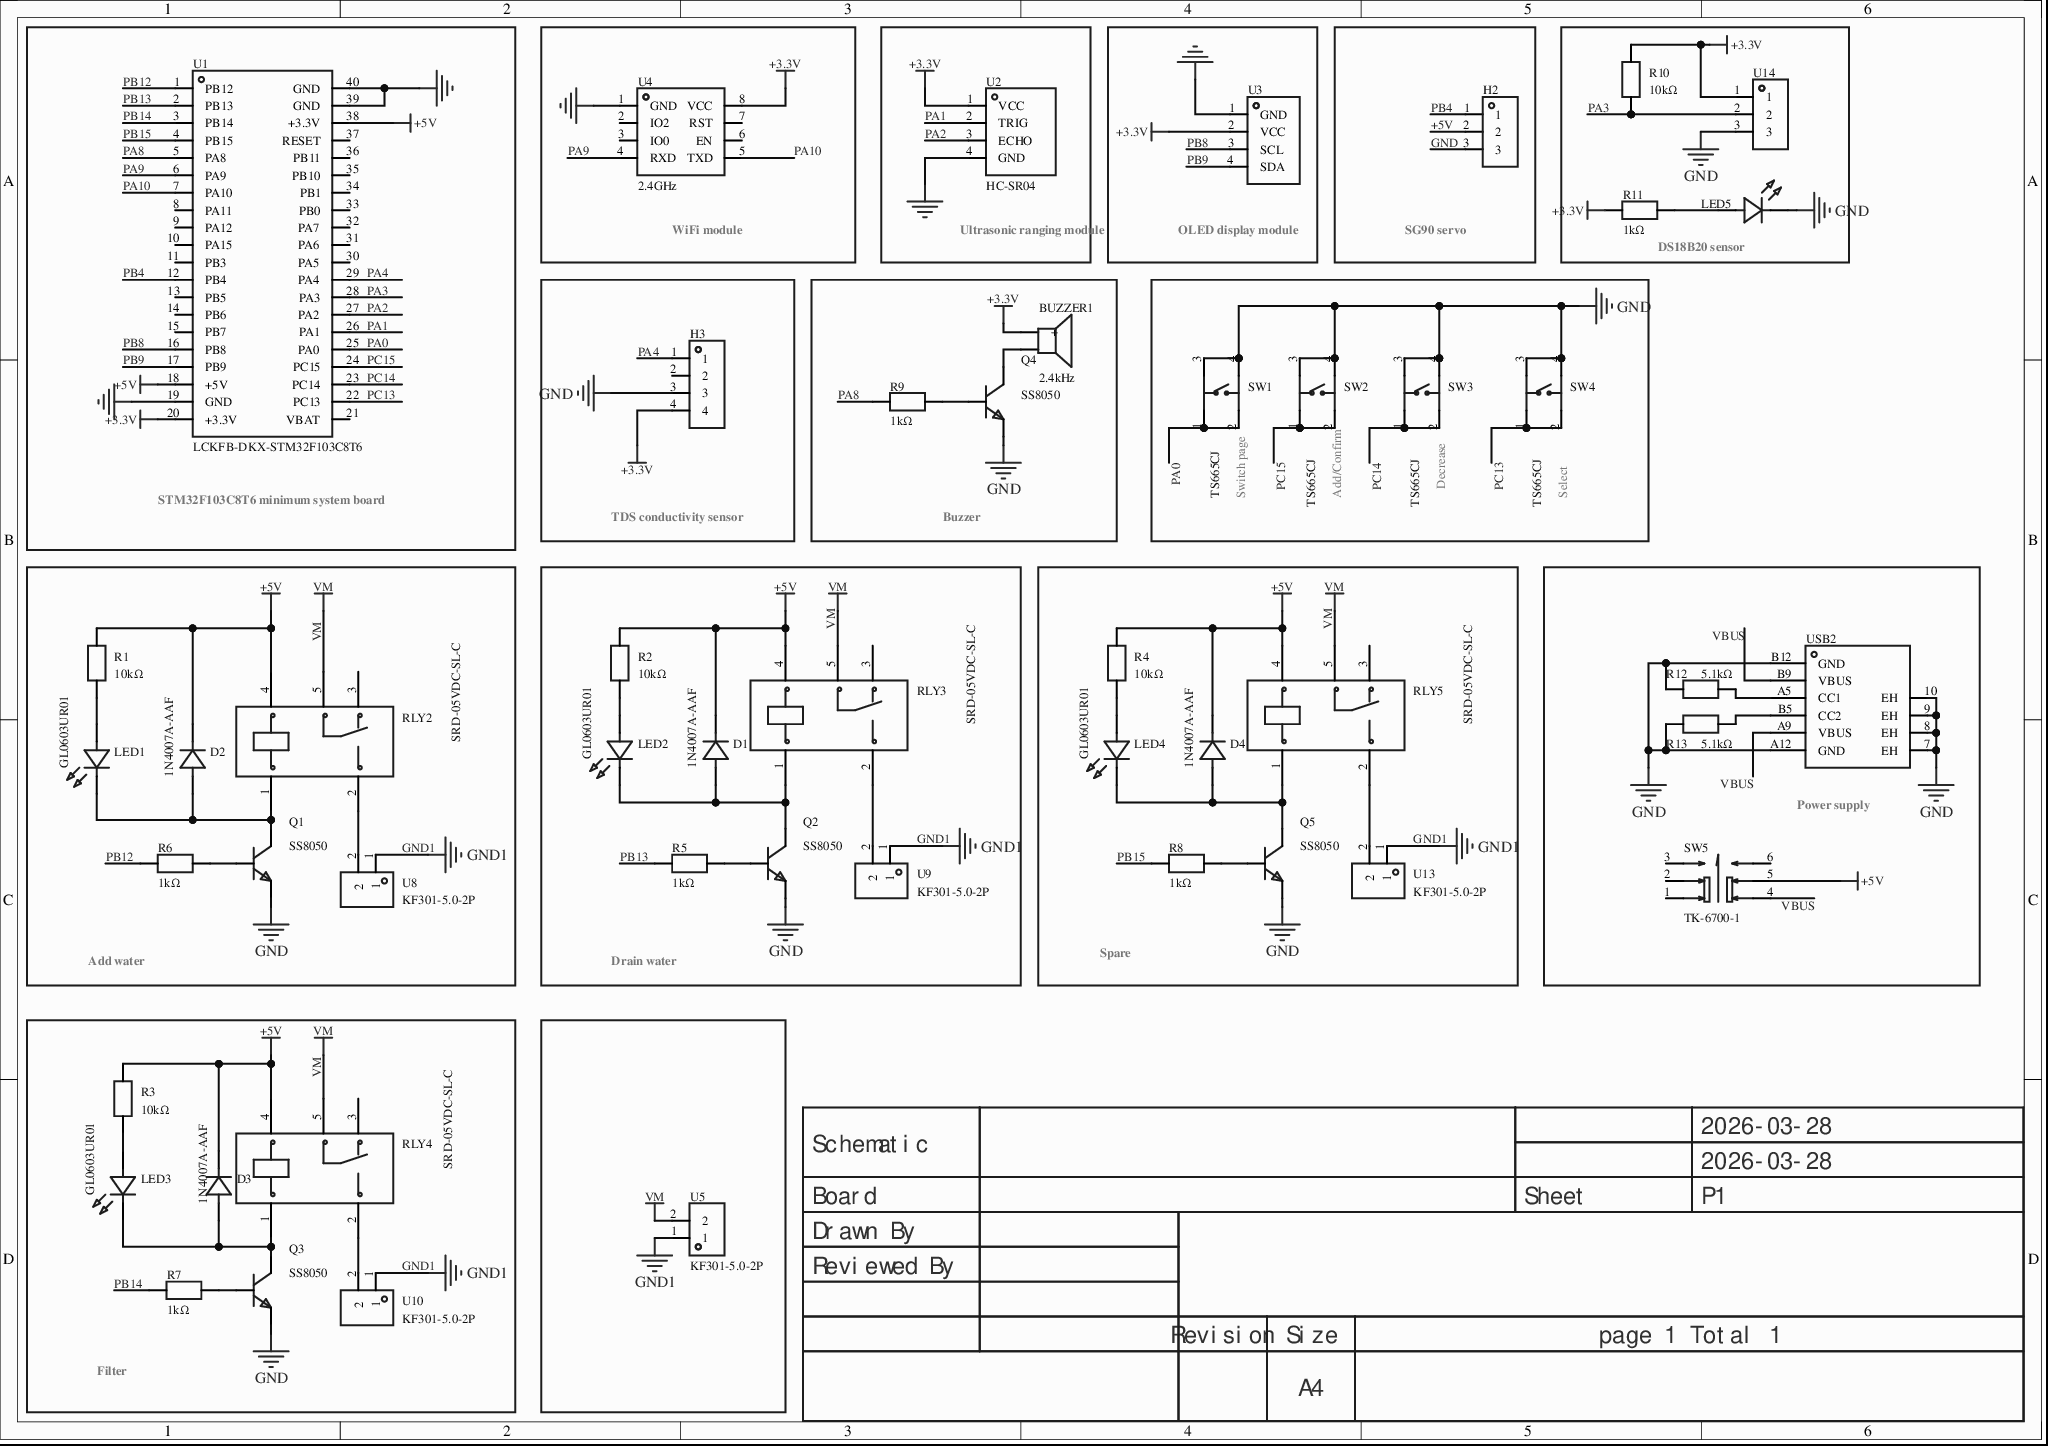
[diagram p0: MISC62342-3.schdoc]
# Altium project MISC62342-2.PrjPcb
1 sheet, 50 parts. Net scope: global (net labels, ports and power ports of the same name join across sheets).
Board file: MISC62342.pcbdoc

## Sheet MISC62342-3.schdoc
size 297 x 209 mm; Version: V1.0; @Project Name: MISC62342; @Page Count: 1; @Update Date: 2026-03-28; @Create Date: 2026-03-28; @Schematic Name: MISC62342; @Page No: 1; @Board Name: MISC62342; @Create Time: 18:09:04; @Update Time: 20:53:11; Size: A4

### Parts
BUZZER1  2.4kHz  [BUZ-TH_BD12.0-P7.60-D0.6-FD]
D1  1N4007A-AAF  [SMA_L4.3-W2.6-LS5.0-RD]
D2  1N4007A-AAF  [SMA_L4.3-W2.6-LS5.0-RD]
D3  1N4007A-AAF  [SMA_L4.3-W2.6-LS5.0-RD]
D4  1N4007A-AAF  [SMA_L4.3-W2.6-LS5.0-RD]
H2  PZ254V-11-03P  [HDR-TH_3P-P2.54-V-M_PZ254V-11-03P]  (value not drawn)
H3  PZ254V-11-04P  [HDR-TH_4P-P2.54-V-M]  (value not drawn)
LED1  GL0603UR01  [LED0603-FD]
LED2  GL0603UR01  [LED0603-FD]
LED3  GL0603UR01  [LED0603-FD]
LED4  GL0603UR01  [LED0603-FD]
LED5  GL0603UR01  [LED0603-FD]  (value not drawn)
Q1  SS8050  [SOT-23-3_L2.9-W1.3-P1.90-LS2.4-BR]
Q2  SS8050  [SOT-23-3_L2.9-W1.3-P1.90-LS2.4-BR]
Q3  SS8050  [SOT-23-3_L2.9-W1.3-P1.90-LS2.4-BR]
Q4  SS8050  [SOT-23-3_L2.9-W1.3-P1.90-LS2.4-BR]
Q5  SS8050  [SOT-23-3_L2.9-W1.3-P1.90-LS2.4-BR]
R1  10kΩ  [RES-TH_BD2.7-L6.2-P10.20-D0.4]
R2  10kΩ  [RES-TH_BD2.7-L6.2-P10.20-D0.4]
R3  10kΩ  [RES-TH_BD2.7-L6.2-P10.20-D0.4]
R4  10kΩ  [RES-TH_BD2.7-L6.2-P10.20-D0.4]
R5  1kΩ  [RES-TH_BD2.7-L6.2-P10.20-D0.4]
R6  1kΩ  [RES-TH_BD2.7-L6.2-P10.20-D0.4]
R7  1kΩ  [RES-TH_BD2.7-L6.2-P10.20-D0.4]
R8  1kΩ  [RES-TH_BD2.7-L6.2-P10.20-D0.4]
R9  1kΩ  [RES-TH_BD2.7-L6.2-P10.20-D0.4]
R10  10kΩ  [RES-TH_BD2.7-L6.2-P10.20-D0.4]
R11  1kΩ  [RES-TH_BD2.7-L6.2-P10.20-D0.4]
R12  5.1kΩ  [RES-TH_BD2.7-L6.2-P10.20-D0.4]
R13  5.1kΩ  [RES-TH_BD2.7-L6.2-P10.20-D0.4]
RLY2  SRD-05VDC-SL-C  [RELAY-TH_SRD-XXVDC-XL-C]
RLY3  SRD-05VDC-SL-C  [RELAY-TH_SRD-XXVDC-XL-C]
RLY4  SRD-05VDC-SL-C  [RELAY-TH_SRD-XXVDC-XL-C]
RLY5  SRD-05VDC-SL-C  [RELAY-TH_SRD-XXVDC-XL-C]
SW1  TS665CJ  [SW-TH_4P-L6.0-W6.0-P4.50-LS6.5]
SW2  TS665CJ  [SW-TH_4P-L6.0-W6.0-P4.50-LS6.5]
SW3  TS665CJ  [SW-TH_4P-L6.0-W6.0-P4.50-LS6.5]
SW4  TS665CJ  [SW-TH_4P-L6.0-W6.0-P4.50-LS6.5]
SW5  TK-6700-1  [SW-TH_TK-6700-1]
U1  LCKFB-DKX-STM32F103C8T6  [CONN-TH_L53.3-W22.9_STM32F103C8T6-CARD]
U2  HC-SR04  [TH_HC-SR04V]
U3  HS96L03W2C03  [OLED-TH_L27.8-W27.2-P2.54_C9900033791]  (value not drawn)
U4  2.4GHz  [WIFIM-TH_8P-L24.7-W14.4-P2.54]
U5  KF301-5.0-2P  [CONN-TH_P5.00_KF301-5.0-2P]
U8  KF301-5.0-2P  [CONN-TH_P5.00_KF301-5.0-2P]
U9  KF301-5.0-2P  [CONN-TH_P5.00_KF301-5.0-2P]
U10  KF301-5.0-2P  [CONN-TH_P5.00_KF301-5.0-2P]
U13  KF301-5.0-2P  [CONN-TH_P5.00_KF301-5.0-2P]
U14  WAFER-XH2.54-3PWZ  [CONN-TH_3P-P2.50_WAFER-XH2.54-3PWZ]  (value not drawn)
USB2  (no value)  [USB_ TYPE-C-6P]

### Blocks framed on the sheet
STM32F103C8T6 minimum system board: U1
WiFi module: U4
Ultrasonic ranging module: U2
OLED display module: U3
SG90 servo: H2
DS18B20 sensor: LED5 R10 R11 U14
TDS conductivity sensor: H3
Buzzer: BUZZER1 Q4 R9
Add water: D2 LED1 Q1 R1 R6 RLY2 U8
Drain water: D1 LED2 Q2 R2 R5 RLY3 U9
Spare: D4 LED4 Q5 R4 R8 RLY5 U13
Power supply: R12 R13 SW5 USB2
Filter: D3 LED3 Q3 R3 R7 RLY4 U10

### Nets
+3.3V: BUZZER1.1(+) H3.4 R10.2 R11.2 U1.20(+3.3V) U2.1(VCC) U3.2(VCC) U4.8(VCC) U14.1
+5V: D1.1(K) D2.1(K) D3.1(K) D4.1(K) H2.2 R1.2 R2.2 R3.2 R4.2 RLY2.4 RLY3.4 RLY4.4 RLY5.4 SW5.5 U1.18(+5V) U1.38(+3.3V)
GND: H2.3 H3.3 LED5.1(K) Q1.2(E) Q2.2(E) Q3.2(E) Q4.2(E) Q5.2(E) R12.1 R13.2 SW1.3(B) SW1.4(D) SW2.3(B) SW2.4(D) SW3.3(B) SW3.4(D) SW4.3(B) SW4.4(D) U1.19(GND) U1.39(GND) U1.40(GND) U2.4(GND) U3.1(GND) U4.1(GND) U14.3 USB2.7(EH) USB2.8(EH) USB2.9(EH) USB2.10(EH) USB2.A12(GND) USB2.B12(GND)
GND1: U5.1 U8.1 U9.1 U10.1 U13.1
VM: RLY2.5 RLY3.5 RLY4.5 RLY5.5 U5.2
PA0: SW1.1(A) SW1.2(C) U1.25(PA0)
PA1: U1.26(PA1) U2.2(TRIG)
PA2: U1.27(PA2) U2.3(ECHO)
PA3: R10.1 U1.28(PA3) U14.2
PA4: H3.1 U1.29(PA4)
PA8: R9.1 U1.5(PA8)
PA9: U1.6(PA9) U4.4(RXD)
PA10: U1.7(PA10) U4.5(TXD)
PB4: H2.1 U1.12(PB4)
PB8: U1.16(PB8) U3.3(SCL)
PB9: U1.17(PB9) U3.4(SDA)
PB12: R6.1 U1.1(PB12)
PB13: R5.1 U1.2(PB13)
PB14: R7.1 U1.3(PB14)
PB15: R8.1 U1.4(PB15)
PC13: SW4.1(A) SW4.2(C) U1.22(PC13)
PC14: SW3.1(A) SW3.2(C) U1.23(PC14)
PC15: SW2.1(A) SW2.2(C) U1.24(PC15)
VBUS: SW5.4 USB2.A9(VBUS) USB2.B9(VBUS)
NetBUZZER1_2: BUZZER1.2 Q4.3(C)
NetD1_2: D1.2(A) LED2.1(K) Q2.3(C) RLY3.1
NetD2_2: D2.2(A) LED1.1(K) Q1.3(C) RLY2.1
NetD3_2: D3.2(A) LED3.1(K) Q3.3(C) RLY4.1
NetD4_2: D4.2(A) LED4.1(K) Q5.3(C) RLY5.1
NetLED1_2: LED1.2(A) R1.1
NetLED2_2: LED2.2(A) R2.1
NetLED3_2: LED3.2(A) R3.1
NetLED4_2: LED4.2(A) R4.1
NetLED5_2: LED5.2(A) R11.1
NetQ1_1: Q1.1(B) R6.2
NetQ2_1: Q2.1(B) R5.2
NetQ3_1: Q3.1(B) R7.2
NetQ4_1: Q4.1(B) R9.2
NetQ5_1: Q5.1(B) R8.2
NetR12_2: R12.2 USB2.A5(CC1)
NetR13_1: R13.1 USB2.B5(CC2)
NetRLY2_2: RLY2.2 U8.2
NetRLY3_2: RLY3.2 U9.2
NetRLY4_2: RLY4.2 U10.2
NetRLY5_2: RLY5.2 U13.2

Not connected (* = marked no-connect by the designer): H3 2*; RLY2 3*; RLY3 3*; RLY4 3*; RLY5 3*; SW5 1* 2* 3* 6*; U1 8(PA11)* 9(PA12)* 10(PA15)* 11(PB3)* 13(PB5)* 14(PB6)* 15(PB7)* 21(VBAT)* 30(PA5)* 31(PA6)* 32(PA7)* 33(PB0)* 34(PB1)* 35(PB10)* 36(PB11)* 37(RESET)*; U4 2(IO2)* 3(IO0)* 6(EN)* 7(RST)*

### Notes on the sheet
- (near SW1) Switch page
- (near SW2) Add/Confirm
- (near SW3) Decrease
- (near SW4) Select
- 2026-03-28
- Schematic
- Board
- Sheet
- P1
- Drawn By
- Reviewed By
- Revision
- Size
- A4
- page 1 Total 1

### Library data of the parts
BUZZER1 = TMB12A05_C96093: Drive mode: Active (built-in driver circuit); Construction: Electromagnetic; Rated voltage: 5V; Frequency: 2.4kHz; Sound pressure (SPL): 85dB;; Manufacturer: 华能; AddInBom: yes; ModelId: 16ab50e14c5b4f2c986c135bdba60e37; ModelName: BUZ-TH_D12.0-H9.5-P7.60; ModelTransform: 472.44,472.176,0,90,0,0,-0.787,0,-177.165; Voltage - Supply: 4V~8V; Current Consumption: 30mA; Symbol: TMB12A05; Device: TMB12A05_C96093; LCSC Part Name: 有源(内含驱动线路) 电磁式 2.4kHz; SupplierPart: C96093; ManufacturerPart: TMB12A05; Supplier Footprint: 插件,D=12mm; JLCPCB Part Class: Extended Library; Datasheet: example.com/datasheet/TMB12A05/97297.html; Supplier: LCSC; ConvertToPcb: yes; FootprintName: BUZ-TH_BD12.0-P7.60-D0.6-FD; Driver Circuitry: Active (built-in driver circuit); Technology: Electromagnetic; Voltage Rating: 5V; Value: 2.4kHz; Sound Pressure Level(SPL): 85dB; Diameter(φD): 12mm; Length: -; Width: -; Height: 9.8mm; Operating Temperature: -40℃~+85℃
D1-D4 = 1N4007A-AAF: Diode configuration: Discrete; Forward voltage (Vf): 1.1V@1A; DC reverse voltage (Vr): 1kV; Rectifier current: 1A;; Manufacturer: FOSAN(富捷/富信); AddInBom: yes; ModelId: 8d2dd2e50a3a4b27821fa63d469a8f11; ModelTransform: 196.85,102.362,0,0,0,0,0,0,0; Reverse Leakage Current (Ir): 5uA; Non-Repetitive Peak Forward Surge Current: 30A; Operating Junction Temperature Range: -65℃~+150℃; Symbol: 1N4007A-AAF; Device: 1N4007A-AAF; LCSC Part Name: 1kV 1A; SupplierPart: C48947090; ManufacturerPart: 1N4007A-AAF; Supplier Footprint: SMA(DO-214AC); JLCPCB Part Class: Extended Library; Datasheet: example.com/datasheet/1N4007A-AAF/51267526.html; Supplier: LCSC; ConvertToPcb: yes; FootprintName: SMA_L4.3-W2.6-LS5.0-RD; ModelName: SMA_L4.3-W2.6-LS5.0-RD; Diode Configuration: Discrete; Voltage - Forward(Vf@If): 1.1V@1A; Voltage - DC Reverse(Vr): 1kV; Current - Rectified: 1A
H2 = PZ254V-11-03P: Pin structure: 1x3P; Pitch: 2.54mm; Row spacing: -; Round/square pin: Square pin; Mounting: Through-hole; Rows: Single row; Total pin count: 3P; Rated current: 3A; Rated voltage: 250V; Mating pin length: 6mm; Plastic height: 2.5mm; Termination pin length: 3mm; Operating temperature: -40℃~+105℃; Color: Black;; Manufacturer: XFCN(兴飞); Symbol: MDF7-3P-2.54DSA(95); AddInBom: yes; ModelId: bb473b6d38ff42a99216a4fcdbdcc4cb; ModelName: HDR-TH_3P-P2.54-M-LI-1X3P; ModelTransform: 300.03877,100,0,0,0,0,0,0,-118.11; Device: PZ254V-11-03P; LCSC Part Name: 1x3P 间距:2.54mm 方针 直插; SupplierPart: C2937625; ManufacturerPart: PZ254V-11-03P; Supplier Footprint: 插件,P=2.54mm; JLCPCB Part Class: Extended Part; Datasheet: example.com/datasheet/PZ254V-11-03P/3293280.html; Supplier: LCSC; ConvertToPcb: yes; FootprintName: HDR-TH_3P-P2.54-V-M_PZ254V-11-03P; Pin Structure: 1x3P; Row Spacing: -; Circluar Pins/Square Pins: Square pin; Mounting Type: Through-hole; Number of Rows: Single row; Number of Pins: 3P; Current Rating: 3A; Voltage Rating (Max): 250V; Length of Mating Pin: 6mm; Insulation Height: 2.5mm; Length of End Connection Pin: 3mm; Operating Temperature: -40℃~+105℃; Color: Black
H3 = PZ254V-11-04P: Pin structure: 1x4P; Pitch: 2.54mm; Row spacing: -; Round/square pin: Square pin; Mounting: Through-hole; Rows: Single row; Total pin count: 4P; Rated current: 3A; Rated voltage: 250V; Mating pin length: 6mm; Plastic height: 2.5mm; Termination pin length: 3mm; Contact material: -; Operating temperature: -40℃~+105℃; Color: Black;; Manufacturer: XFCN(兴飞); Symbol: PZ254V-11-04P_C2691448; AddInBom: yes; ModelId: 112f4d05e8d64e99ab9a333894bea4f9; ModelName: HDR-TH_4P-P2.54-M-LI-1X4P; ModelTransform: 399.999,104.7242,0,0,0,0,0,0,-118.11; Device: PZ254V-11-04P; LCSC Part Name: 1x4P 间距:2.54mm 方针 直插; SupplierPart: C2691448; ManufacturerPart: PZ254V-11-04P; Supplier Footprint: 插件,P=2.54mm; JLCPCB Part Class: Extended Library; Datasheet: example.com/datasheet/PZ254V-11-04P/2801085.html; Supplier: LCSC; ConvertToPcb: yes; FootprintName: HDR-TH_4P-P2.54-V-M; Pin Structure: 1x4P; Row Spacing: -; Circluar Pins/Square Pins: Square pin; Mounting Type: Through-hole; Number of Rows: Single row; Number of Pins: 4P; Current Rating: 3A; Voltage Rating (Max): 250V; Length of Mating Pin: 6mm; Insulation Height: 2.5mm; Length of End Connection Pin: 3mm; Contact Material: -; Operating Temperature: -40℃~+105℃; Color: Black
LED1-LED5 = GL0603UR01: Emitting color: Red; Forward voltage (Vf): 2.4V; Forward current: 20mA; Wavelength: 620nm~625nm; Diode configuration: Discrete diode; Lens color: Clear lens; Luminous intensity: 120mcd; Viewing angle: 120°; Packaging: Surface mount; Operating temperature: -40℃~+85℃;; Manufacturer: Guiguang light(桂光光电); Symbol: 3A2RUD; AddInBom: yes; ModelId: b57d6965da4c4e30afc1a994a1f136ae; ModelName: LED0603_Inf; ModelTransform: 60,30,0,0,0,0,0,0,0; Device: GL0603UR01; LCSC Part Name: 0603 红灯 高亮; SupplierPart: C51933292; ManufacturerPart: GL0603UR01; Supplier Footprint: 0603; JLCPCB Part Class: Extended Part; Datasheet: example.com/datasheet/GL0603UR01/54645988.html; Supplier: LCSC; ConvertToPcb: yes; FootprintName: LED0603-FD; Illumination Color: Red; Voltage - Forward(Vf): 2.4V; Forward Current: 20mA; Wavelength - Dominant: 620nm~625nm; Diode Configuration: Discrete diode; Lens Color: Clear lens; Luminous Intensity: 120mcd; Viewing Angle: 120°; Mounting Style: Surface mount; Operating Temperature: -40℃~+85℃
Q1-Q5 = SS8050_C7420370: Transistor type: NPN; Collector current (Ic): 1.5A; Collector-emitter breakdown voltage (Vceo): 25V; Power dissipation (Pd): 300mW; DC current gain (hFE): 120@100mA,1.0V;; Manufacturer: R+O(宏嘉诚); AddInBom: yes; ModelId: c62791f0466c4ae2a892c056b845b0ca; ModelName: SOT-23-3P_L2.9-W1.3-H1.0-LS2.4-P0.95; ModelTransform: 98.425,114.173,0,180,0,0,0.0005,-0.0005,0; Transition frequency(fT): 100MHz; Current - Collector Cutoff: 100nA; Vce Saturation(VCE(sat)): 500mV; Emitter-Base Voltage(Vebo): 5V; Symbol: SS8050_C7420370; Device: SS8050_C7420370; LCSC Part Name: H档 200-350 NPN 电流:1.5A 电压:25V; SupplierPart: C7420370; ManufacturerPart: SS8050; Supplier Footprint: SOT-23; JLCPCB Part Class: Extended Library; Datasheet: example.com/datasheet/SS8050/8397192.html; Supplier: LCSC; ConvertToPcb: yes; FootprintName: SOT-23-3_L2.9-W1.3-P1.90-LS2.4-BR; type: NPN; Current - Collector(Ic): 1.5A; Collector - Emitter Voltage VCEO: 25V; Pd - Power Dissipation: 300mW; DC Current Gain: 120@100mA,1.0V; Operating Temperature: -55℃~+150℃
R1-R4 R10-R13 = MF1/4W-10K±1%-ST52: Resistor type: Metal film resistor; Resistance: 10kΩ; Tolerance: ±1%; Power: 250mW; Temperature coefficient: ±100ppm/℃;; Manufacturer: VO(翔胜); AddInBom: yes; ModelId: f91fbe0e2e6f409498f09f811e4616fe; ModelTransform: 417.322,106.221,0,0,0,0,0,0,-196.85; Voltage-Supply(Max): 250V; Symbol: MF1/4W-10K±1%-ST52; Device: MF1/4W-10K±1%-ST52; LCSC Part Name: 金属膜电阻 10kΩ ±1% 250mW; ManufacturerPart: MF1/4W-10K±1%-ST52; Supplier Footprint: 插件,D2.7xL6.2mm; JLCPCB Part Class: Extended Library; Datasheet: example.com/datasheet/MF1%252F4W-10K%25C2%25B11%2525-ST52/3158983.html; Supplier: LCSC; ConvertToPcb: yes; FootprintName: RES-TH_BD2.7-L6.2-P10.20-D0.4; ModelName: RES-TH_BD2.7-L6.2-P10.20-D0.4; Type: Metal film resistor; Power(Watts): 250mW; Temperature Coefficient: ±100ppm/℃; Operating Temperature: -55℃~+155℃
  R1-R4 R10: SupplierPart: C2903232; Value: 10kΩ
  R11: Value: 1kΩ
  R12 R13: Value: 5.1kΩ
R5-R9 = MF1/4W-1K±1%-ST52: Resistor type: Metal film resistor; Resistance: 1kΩ; Tolerance: ±1%; Power: 250mW; Temperature coefficient: ±100ppm/℃;; Manufacturer: VO(翔胜); AddInBom: yes; ModelId: f91fbe0e2e6f409498f09f811e4616fe; ModelTransform: 417.322,106.221,0,0,0,0,0,0,-196.85; Voltage-Supply(Max): 250V; Symbol: MF1/4W-1K±1%-ST52; Device: MF1/4W-1K±1%-ST52; LCSC Part Name: 金属膜电阻 1kΩ ±1% 250mW; SupplierPart: C2903245; ManufacturerPart: MF1/4W-1K±1%-ST52; Supplier Footprint: 插件,D2.7xL6.2mm; JLCPCB Part Class: Extended Library; Datasheet: example.com/datasheet/MF1%252F4W-1K%25C2%25B11%2525-ST52/3158996.html; Supplier: LCSC; ConvertToPcb: yes; FootprintName: RES-TH_BD2.7-L6.2-P10.20-D0.4; ModelName: RES-TH_BD2.7-L6.2-P10.20-D0.4; Type: Metal film resistor; Value: 1kΩ; Power(Watts): 250mW; Temperature Coefficient: ±100ppm/℃; Operating Temperature: -55℃~+155℃
RLY2-RLY5 = SRD-05VDC-SL-C: Coil voltage: 5V; Contact form: Changeover: 1C (SPDT); Contact rating (resistive load): -; Max switching voltage: 250V@AC; Max switching current: 15A;; Manufacturer: 松乐; AddInBom: yes; ModelId: d0eda9b8bf8746d18ae810ab88dc78e7; ModelName: RELAY-TH_L19.2-W15.6-H15.8; ModelTransform: 755.904,622.4397,0,0,0,0,34.882,0,-118.11; Coil Rated Power: 360mW; Coil Type: Non-polar, single coil; Coil Resistance: 70Ω; Contact Resistance: 100mΩ; Operate Time: 10ms; Symbol: SRD-05VDC-SL-C; Device: SRD-05VDC-SL-C; LCSC Part Name: 蓝色 单组转换型继电器; SupplierPart: C35449; ManufacturerPart: SRD-05VDC-SL-C; Supplier Footprint: 插件,15.6x19.2mm; JLCPCB Part Class: Extended Library; Datasheet: example.com/datasheet/SRD-05VDC-SL-C/36422.html; Supplier: LCSC; ConvertToPcb: yes; FootprintName: RELAY-TH_SRD-XXVDC-XL-C; Coil Voltage: 5V; Contact Form: Changeover: 1C (SPDT); Number of Pins: 5; Contact Rating: -; Switching Voltage(Max): 250V@AC; Switching Current(Max): 15A; Release Time: 10ms
SW1-SW4 = TS665CJ: Circuit structure: SPST; Button shape: Round button; Actuating force: 2.5N; Mounting: Through-hole; Switch length: 6mm; Switch width: 6mm; Switch height: 5mm; Bracket: Without bracket; Contact current: 50mA; Rated voltage: 12V; Lamp: None; Life: 5万 cycles;; Manufacturer: SHOU HAN(首韩); Symbol: KH-6X6X4.3H-STM; AddInBom: yes; ModelId: 20eee248bc684ccd8cbdbb1d0d91ec6f; ModelName: SW-TH_4P-L6.0-W6.0-H5.0-LS6.5-P4.50; ModelTransform: 236.22,323.03,0,90,0,0,0,0,-137.795; Actuator/Cap Color: Black; JLCPCB Part Class: Extended Part; Device: TS665CJ; LCSC Part Name: 6*6*5mm 直插 轻触开关; SupplierPart: C393938; ManufacturerPart: TS665CJ; Supplier Footprint: 插件-4P,6x6mm; Datasheet: example.com/datasheet/TS665CJ/372550.html; Supplier: LCSC; ConvertToPcb: yes; FootprintName: SW-TH_4P-L6.0-W6.0-P4.50-LS6.5; Circuit: SPST; Actuator Style: Round button; Operating Force: 2.5N; Mounting Type: Through-hole; Length: 6mm; Width: 6mm; Switch Height: 5mm; with Bracket: Without bracket; Contact Current: 50mA; Voltage Rating: 12V; With Lamp: None; Termination Style: PC pin; Life: 5万 cycles; Operating Temperature: -25℃~+70℃
SW5 = TK-6700-1: Circuit structure: DPDT; Self-locking/unlocking: Self-locking; Mounting: Through-hole; Actuating force: 2.3N; Operating life: -;; Manufacturer: Yuandi(元迪); AddInBom: yes; ModelId: 1dccfbf2ceb24a728093c1f6ee61932a; ModelTransform: 275.59,275.59,0,90,0,0,0,0,-137.795; Actuator Style: Rectangular plunger; Actuator/Cap Color: Blue; Symbol: TK-6700-1; Device: TK-6700-1; LCSC Part Name: 自锁开关7*7*12.7有声有锁高导高柄插件双排6P按键开关带锁DIP六脚; SupplierPart: C528782; ManufacturerPart: TK-6700-1; Supplier Footprint: 插件; JLCPCB Part Class: Extended Library; Datasheet: example.com/datasheet/TK-6700-1/548571.html; Supplier: LCSC; ConvertToPcb: yes; FootprintName: SW-TH_TK-6700-1; ModelName: SW-TH_TK-6700-1; Circuit: DPDT; Self Lock / No Lock: Self-locking; Mounting Type: Through-hole; Termination Style: PC pin; Operating Force: 2.3N; Life: -
U1 = LCKFB-DKX-STM32F103C8T6: Manufacturer: 立创开发板; AddInBom: yes; Symbol: LCKFB-DKX-STM32F103C8T6; Device: LCKFB-DKX-STM32F103C8T6; LCSC Part Name: 立创·地阔星-STM32F103C8T6开发板; SupplierPart: C22396880; ManufacturerPart: LCKFB-DKX-STM32F103C8T6; Supplier Footprint: -; JLCPCB Part Class: Extended Library; Datasheet: example.com/datasheet/LCKFB-DKX-STM32F103C8T6/24005615.html; Supplier: LCSC; ConvertToPcb: yes; FootprintName: CONN-TH_L53.3-W22.9_STM32F103C8T6-CARD
U2 = HC-SR04: Manufacturer: Universal Microelectronics; AddInBom: yes; ModelId: d459d248281f4140aaafbda3f8c1b0d5; Symbol: HC-SR04; Device: HC-SR04; LCSC Part Name: HC-SR04; SupplierPart: C19857336; ManufacturerPart: HC-SR04; Supplier Footprint: -; JLCPCB Part Class: Extended Library; Datasheet: example.com/pdf/source/20240122/47B8E374E428935B7962A2189EF91AAC.pdf; Supplier: LCSC; ConvertToPcb: yes; FootprintName: TH_HC-SR04V; ModelName: HC-SR04
U3 = HS96L03W2C03: Controller chip: SSD1315; Interface type: I2C; Size (inch): 0.96; Pixel resolution: 128x64;; Manufacturer: HS(汉昇); AddInBom: yes; ModelId: bb65183306db4ca69fb52250be49b00e; ModelTransform: 1070.864,1094.486,0,0,0,0,0,-498.424,0; Symbol: HS96L03W2C03; Device: HS96L03W2C03; LCSC Part Name: 0.96寸OLED显示屏窄白光IIC; SupplierPart: C5248080; ManufacturerPart: HS96L03W2C03; Supplier Footprint: -; JLCPCB Part Class: Extended Library; Datasheet: example.com/pdf/source/20230627/763D01F79A90007632F098068C7C8AD9.pdf; Supplier: LCSC; ConvertToPcb: yes; FootprintName: OLED-TH_L27.8-W27.2-P2.54_C9900033791; ModelName: OLED-TH_L27.8-W27.2-P2.54_C9900033791; Main Control Chip: SSD1315; Interface Type: I2C; Size: 0.96; Pixel Resolution: 128x64; Operating Temperature: -40℃~+70℃
U4 = ESP-01S: Core processor: ESP8266 chip; Frequency: 2.4GHz; Antenna type: On-board PCB antenna; TX power: 16dBm; RX sensitivity: -90dBm;; Manufacturer: Ai-Thinker(安信可); Symbol: ESP-01S_C503582; AddInBom: yes; ModelId: 9453774c1eaa4779b246df5901e96246; ModelName: WIFIM-TH_8P-L24.7-W14.4-H2.8-P2.54; ModelTransform: 972.43904,566.928,0,0,0,0,377.167,-3.936,-118.11; Support Interface: GPIO; UART; PWM; Operating Voltage: 3V~3.6V; Receive  Current: 56mA; Send  Current: 170mA; Device: ESP-01S; LCSC Part Name: 完整的802.11b/g/nWi-FiSoC模块; SupplierPart: C503582; ManufacturerPart: ESP-01S; Supplier Footprint: -; JLCPCB Part Class: Extended Library; Datasheet: example.com/pdf/source/20200407/C503582_1139AF8FB42E05635FA0089E1752A536.pdf; Supplier: LCSC; ConvertToPcb: yes; FootprintName: WIFIM-TH_8P-L24.7-W14.4-P2.54; Core Processor: ESP8266 chip; Wireless Standard: -; Value: 2.4GHz; Antenna Type: On-board PCB antenna; Output Power: 16dBm; Sensitivity: -90dBm; Operating Temperature: -20℃~+70℃
U5 = KF301-5.0-2P: Structure: 1x2P; Pitch: 5mm; Color: Blue; Mounting: Through-hole; Rows: 1; Pins per row: 2; Rated current: 17A; Rated voltage: 250V; Wire gauge - AWG: 14~22; Wire gauge - mm²: 1.5; Operating temperature: -30℃~+120℃;; Manufacturer: KEFA(科发); 3D Model: 442de893d0fc4728b9e5c7abc29ccda5; 3D Model Transform: 417.322,299.21594,0,0,0,0,11.811,7.874,-137.795; Number of PINs Per Row: 2; Wire Gauge - mm2: 1.5; AddInBom: yes; Symbol: KF301-5.0-2P; Device: KF301-5.0-2P; LCSC Part Name: 1x2P 5mm 直插 排数:1 每排P数:2; Supplier Part: C474881; Manufacturer Part: KF301-5.0-2P; Supplier Footprint: 插件,P=5mm; JLCPCB Part Class: Extended Library; Datasheet: example.com/datasheet/KF301-5.0-2P/481499.html; Supplier: LCSC; Number of Positions or Pins: 1x2P; Mounting Type: Through-hole; Number of Pins: 2P; Number of Rows: 1; Current Rating: 17A; Voltage Rating (Max): 250V; Wire Gauge - AWG: 14~22; Operating Temperature: -30℃~+120℃; ConvertToPcb: yes; FootprintName: CONN-TH_P5.00_KF301-5.0-2P; ModelName: CONN-TH_P5.00_KF301-5.0-2P
U8-U10 U13 = KF301-5.0-2P: Structure: 1x2P; Pitch: 5mm; Color: Blue; Mounting: Through-hole; Rows: 1; Pins per row: 2; Rated current: 17A; Rated voltage: 250V; Wire gauge - AWG: 14~22; Wire gauge - mm²: 1.5; Operating temperature: -30℃~+120℃;; Manufacturer: KEFA(科发); AddInBom: yes; ModelId: 442de893d0fc4728b9e5c7abc29ccda5; ModelTransform: 417.322,299.21594,0,0,0,0,11.811,7.874,-137.795; Number of PINs Per Row: 2; Wire Gauge - mm2: 1.5; Symbol: KF301-5.0-2P; Device: KF301-5.0-2P; LCSC Part Name: 1x2P 5mm 直插 排数:1 每排P数:2; SupplierPart: C474881; ManufacturerPart: KF301-5.0-2P; Supplier Footprint: 插件,P=5mm; JLCPCB Part Class: Extended Library; Datasheet: example.com/datasheet/KF301-5.0-2P/481499.html; Supplier: LCSC; ConvertToPcb: yes; FootprintName: CONN-TH_P5.00_KF301-5.0-2P; ModelName: CONN-TH_P5.00_KF301-5.0-2P; Number of Positions or Pins: 1x2P; Mounting Type: Through-hole; Number of Pins: 2P; Number of Rows: 1; Current Rating: 17A; Voltage Rating (Max): 250V; Wire Gauge - AWG: 14~22; Operating Temperature: -30℃~+120℃
U14 = WAFER-XH2.54-3PWZ: Pin structure: 1x3P; Pitch: 2.5mm; Mounting: Right angle; Reference series: XH; Total pin count: 3P; Rows: 1; Pins per row: 3; Row spacing: -; Rated current: 2A; Contact material: Brass; Contact plating: Tin; Operating temperature: -25℃~+85℃;; Manufacturer: XUNPU(讯普); AddInBom: yes; ModelId: 964060380ab84c59b2a38cefb7706dab; ModelTransform: 394.094,300.7868,0,0,0,0,-0.005,-137.795,-133.858; Number of PINs Per Row: 3; Voltage Rating: 250V; Plastic Material: PA66; Flame Retardant Rating: UL94V-0; Z-Height of the Board: 5.9mm; X-Length of Bottom Edge on Board (Spacing Line): 10mm; Y-Width of Bottom Edge on Board: 7.32mm; Symbol: WAFER-XH2.54-3PWZ; Device: WAFER-XH2.54-3PWZ; LCSC Part Name: 1x3P 间距:2.5mm 弯插 系列:XH; SupplierPart: C5374806; ManufacturerPart: WAFER-XH2.54-3PWZ; Supplier Footprint: 弯插,P=2.5mm; JLCPCB Part Class: Extended Library; Datasheet: example.com/datasheet/WAFER-XH2.54-3PWZ/6231118.html; Supplier: LCSC; ConvertToPcb: yes; FootprintName: CONN-TH_3P-P2.50_WAFER-XH2.54-3PWZ; ModelName: CONN-TH_3P-P2.50_WAFER-XH2.54-3PWZ; Pins Structure: 1x3P; Mounting Type: Right angle; Reference Series: XH; Number of Pins: 3P; Number of Rows: 1; Row Spacing: -; Current Rating: 2A; Contact Material: Brass; Contact Plating: Tin; Operating Temperature: -25℃~+85℃; Supplementary Features: -; Color: White
USB2 = USB_ Type-C-6P: AddInBom: yes; ModelId: d4f492a4e6024845a13b3f6a4ef2d2cb; ModelName: USB-SMD_U262-061N-4BVC11; ModelTransform: 352.362,281.496,0,0,0,0,0,-47.244,-39.37; Device: USB_ Type-C-6P; Supplier Footprint: SMD; ConvertToPcb: yes; SymbolName: USB_ TYPE-C-6P; FootprintName: USB_ TYPE-C-6P